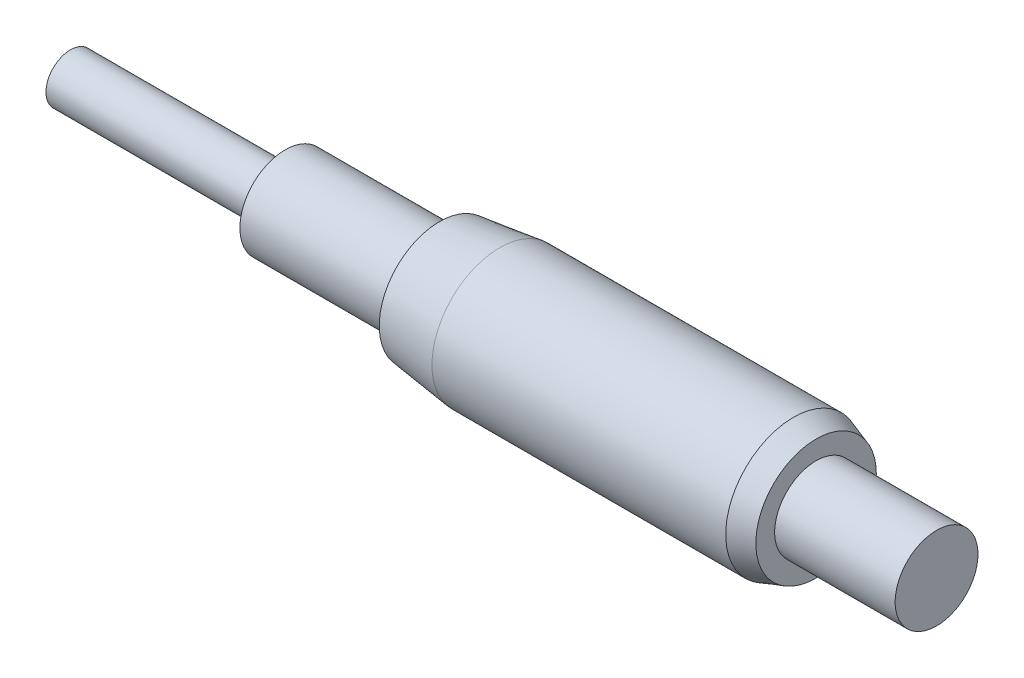
from build123d import *


with BuildPart() as part:
    # Sketch1 → Revolve1 (revolve)
    with BuildSketch(Plane.XY, mode=Mode.PRIVATE) as revolve1_sk:
        Polygon((28.5, 3.25), (0, 3.25), (0, 0), (115, 0), (115, 5.5), (99, 5.5), (99, 8), (96, 9), (57, 9), (49, 8), (49, 6), (28.5, 6), align=None)
    revolve(revolve1_sk.sketch.rotate(Axis((115, 0, 0), (-1, 0, 0)), 90), axis=Axis((115, 0, 0), (-1, 0, 0)))


solid = part.part
